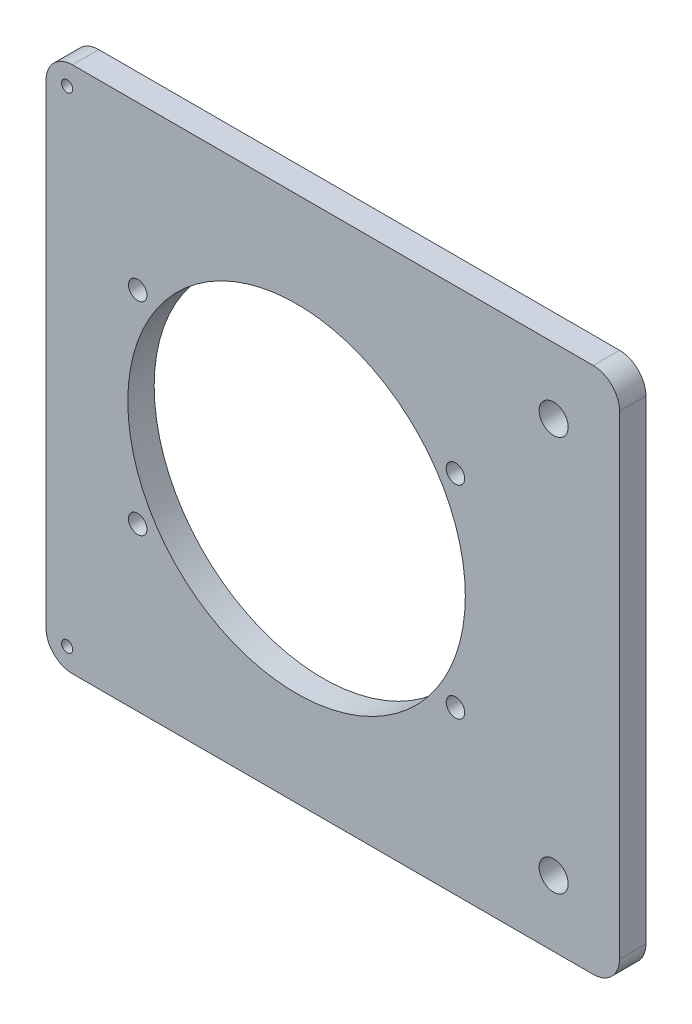
SolidWorks part; units mm, degrees
material "AISI 304"
ref_plane "Front Plane" through (0, 0, 0) normal (0, 0, 1) x (1, 0, 0)
ref_plane "Top Plane" through (0, 0, 0) normal (0, 1, 0) x (1, 0, 0)
ref_plane "Right Plane" through (0, 0, 0) normal (1, 0, 0) x (0, 0, -1)
sketch "Sketch1" plane through (0, 0, 0) normal (0, 0, 1) x (1, 0, 0)
  line L1 (-95, -100) -> (95, -100)
  line L2 (-95, -100) -> (-95, 100)
  line L3 (-95, 100) -> (95, 100)
  line L4 (95, -100) -> (95, 100)
  line L5 (-95, -100) -> (95, 100) construction
  line L6 (-95, 100) -> (95, -100) construction
  point P0 (0, 0)
  dimension "D1" = 190
  dimension "D2" = 200
extrude "Boss-Extrude1" add sketch "Sketch1" along normal blind 10
sketch "Sketch2" plane through (0, 0, 10) normal (0, 0, 1) x (1, 0, 0)
  circle A0 centre (0, 0) radius 64
  dimension "D1" = 128
extrude "Cut-Extrude1" cut sketch "Sketch2" against normal up to surface (10 mm away) up to face at (0, 0, 0)
sketch "Sketch3" plane through (0, 0, 10) normal (0, 0, 1) x (1, 0, 0)
  line L0 (0, 0) -> (0, 150.4955) construction
  line L1 (0, 0) -> (-150.6467, 0) construction
  circle A0 centre (-60.25, 38.425) radius 3.5
  circle A1 centre (60.25, 38.425) radius 3.5
  circle A2 centre (60.25, -38.425) radius 3.5
  circle A3 centre (-60.25, -38.425) radius 3.5
extrude "Cut-Extrude2" cut sketch "Sketch3" against normal blind 10
sketch "Sketch4" plane through (0, 0, 10) normal (0, 0, 1) x (1, 0, 0)
  line L0 (95, 100) -> (-95, 100) construction
  line L1 (95, -100) -> (122.5, -100)
  line L2 (95, -100) -> (95, 100)
  line L3 (95, 100) -> (122.5, 100)
  line L4 (122.5, -100) -> (122.5, 100)
  dimension "D1" = 27.5
extrude "Boss-Extrude2" add sketch "Sketch4" against normal blind 10
sketch "Sketch5" plane through (0, 0, 10) normal (0, 0, 1) x (1, 0, 0)
  line L0 (0, 0) -> (222.0843, 0) construction
  line L1 (122.5, -100) -> (122.5, 100) construction
  line L2 (122.5, 100) -> (-95, 100) construction
  circle A0 centre (97.5, 75) radius 5.5
  circle A1 centre (97.5, -75) radius 5.5
  dimension "D1" = 11
  dimension "D2" = 25
  dimension "D3" = 25
extrude "Cut-Extrude3" cut sketch "Sketch5" against normal blind 10
sketch "Sketch6" plane through (0, 0, 10) normal (0, 0, 1) x (1, 0, 0)
  line L0 (-95, 100) -> (-95, -100) construction
  line L1 (-95, -100) -> (122.5, -100) construction
  line L2 (0, 0) -> (-207.0188, 0) construction
  circle A0 centre (-87, -92) radius 0.5
  circle A1 centre (-87, 92) radius 0.5
  dimension "D1" = 1
  dimension "D2" = 8
  dimension "D3" = 8
extrude "Cut-Extrude4" cut sketch "Sketch6" against normal blind 10
hole_wizard "M5 Tapped Hole1" positions "Sketch7" profile "Sketch8" tap size "M5" standard "GB"
sketch "Sketch7" plane through (0, 0, 10) normal (0, 0, 1) x (1, 0, 0)
  point P0 (-87, 92)
  point P3 (-87, -92)
sketch "Sketch8" plane through (-87, 92, 10) normal (1, 0, 0) x (0, -1, 0)
  line L0 (0, 0) -> (0, 15.2618)
  line L1 (0, 15.2618) -> (2.1, 14)
  line L2 (2.1, 14) -> (2.1, 0)
  line L5 (2.1, 0) -> (0, 0)
  line L10 (0, 15.2618) -> (-2.1, 14) construction
  line L11 (0, -6.35) -> (0, 107.95) construction
  dimension "螺纹孔钻头直径" = 4.2
  dimension "螺纹孔钻头深度" = 14
  dimension "导头角度" = 118
cosmetic thread "Cosmetic Thread1" parameters "D1"=10, "D2"=5
cosmetic thread "Cosmetic Thread2" parameters "D1"=10, "D2"=5
fillet "Fillet1" radius 10 4 edges at (-95, -100, 5) (122.5, 100, 5) (122.5, -100, 5) (-95, 100, 5)
